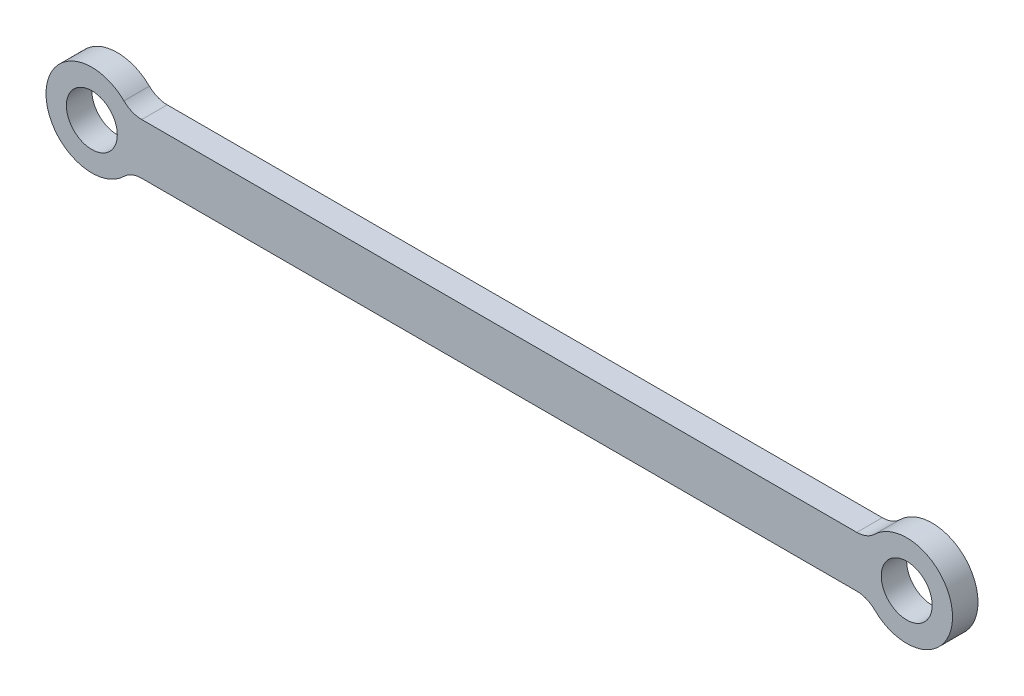
SolidWorks part; units mm, degrees
ref_plane "Front Plane" through (0, 0, 0) normal (0, 0, 1) x (1, 0, 0)
ref_plane "Top Plane" through (0, 0, 0) normal (0, 1, 0) x (1, 0, 0)
ref_plane "Right Plane" through (0, 0, 0) normal (1, 0, 0) x (0, 0, -1)
sketch "Sketch1" plane through (0, 0, 0) normal (0, 0, 1) x (1, 0, 0)
  line L0 (9.798, 5) -> (150.202, 5)
  line L1 (9.798, -5) -> (150.202, -5)
  circle A0 centre (0, 0) radius 5
  arc A1 (6.2987, 6.4286) -> (6.2987, -6.4286) centre (0, 0) ccw
  circle A2 centre (160, 0) radius 5
  arc A3 (153.7013, -6.4286) -> (153.7013, 6.4286) centre (160, 0) ccw
  arc A4 (150.202, 5) -> (153.7013, 6.4286) centre (150.202, 10) ccw
  arc A5 (150.202, -5) -> (153.7013, -6.4286) centre (150.202, -10) cw
  arc A6 (9.798, -5) -> (6.2987, -6.4286) centre (9.798, -10) ccw
  arc A7 (9.798, 5) -> (6.2987, 6.4286) centre (9.798, 10) cw
  dimension "D1" = 10
  dimension "D3" = 18
  dimension "D4" = 5
  dimension "D2" = 160
extrude "Boss-Extrude1" add sketch "Sketch1" along normal blind 5
